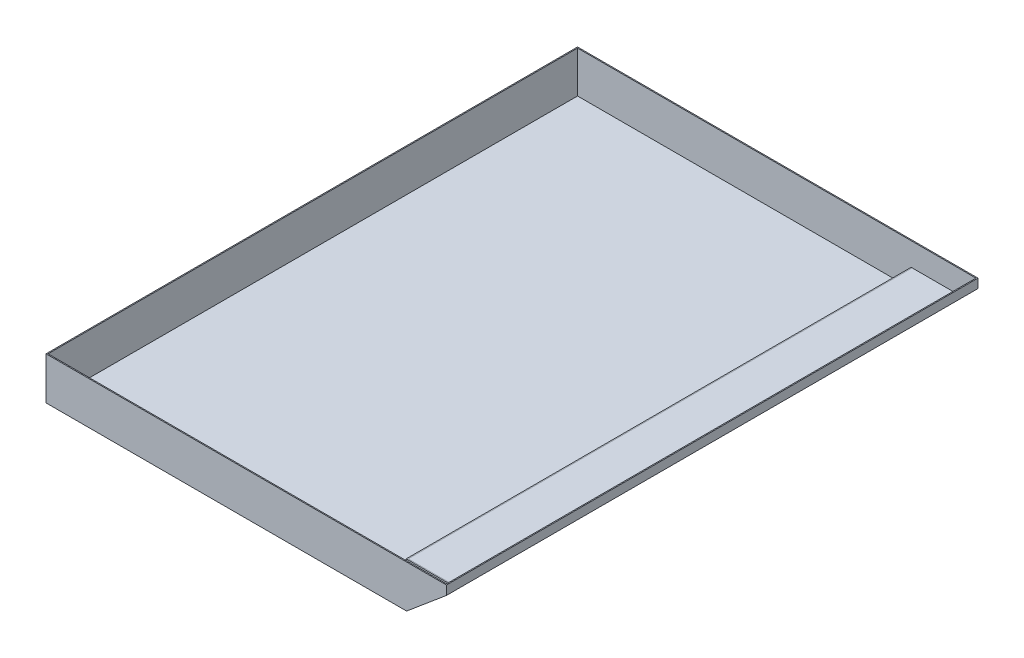
from build123d import *

# Parameters (mm, degrees)
EXTRUDE_1_DEPTH      = 1038
SKETCH_8_W           = 110.00435438
SKETCH_8_H           = 134.15256119
CUT_EXTRUDE_2_DEPTH  = 1191
SHELL_1_T            = -2
SKETCH_3_W           = 75
SKETCH_3_H           = 982
CUT_EXTRUDE_1_DEPTH  = 654
SKETCH_5_W           = 2
SKETCH_5_H           = 986
EXTRUDE_2_DEPTH      = 60
EXTRUDE_3_DEPTH      = 493
EXTRUDE_3_DEPTH_BACK = 493
EXTRUDE_5_DEPTH      = 2
EXTRUDE_6_DEPTH      = 2


with BuildPart() as part:
    # 草图2 → 凸台-拉伸1 (new body)
    with BuildSketch(Plane.XY):
        Polygon((0, 0), (0, 83), (784, 83), (784, 67), (704.152509296, 0), align=None)
    extrude(amount=EXTRUDE_1_DEPTH)

    # 草图8 → 切除-拉伸2 (cut)
    with BuildSketch(Plane.XY.offset(1038)):
        with Locations((837.00217719, 67.076280595)):
            Rectangle(SKETCH_8_W, SKETCH_8_H)
    extrude(amount=-CUT_EXTRUDE_2_DEPTH, mode=Mode.SUBTRACT)

    # 抽壳1
    shell_1_openings = [part.faces().sort_by_distance(p)[0] for p in [
        (391, 83, 519),
    ]]
    offset(amount=SHELL_1_T, openings=shell_1_openings, kind=Kind.INTERSECTION)

    # 草图3 → 切除-拉伸1 (cut)
    with BuildSketch(Plane(origin=(290.938854629, -346.727425229, 0), x_dir=(0.7660444431189772, 0.6427876096865405, 0), z_dir=(0.6427876096865404, -0.7660444431189772, 0))):
        with Locations((590.223457765, 519)):
            Rectangle(SKETCH_3_W, SKETCH_3_H)
    extrude(amount=-CUT_EXTRUDE_1_DEPTH, mode=Mode.SUBTRACT)

    # 草图5 → 凸台-拉伸2 (add)
    with BuildSketch(Plane(origin=(0, 2, 0), x_dir=(1, 0, 0), z_dir=(0, 1, 0))):
        with Locations((678.424568828, -519)):
            Rectangle(SKETCH_5_W, SKETCH_5_H)
    extrude(amount=EXTRUDE_2_DEPTH)


with BuildPart() as body_2:
    # 草图6 → 凸台-拉伸3 (new, two sides: drawn at the far end of the back side and taken through both)
    with BuildSketch(Plane.XY.offset(519).offset(-EXTRUDE_3_DEPTH_BACK)):
        Polygon((679.424568828, 62), (774.929784383, 62), (772.546277198, 60), (681.424568828, 60), (681.424568828, 4), (702.696628359, 4), (746.250437533, 40.545985214), (747.536012752, 39.013896328), (703.424568828, 2), (679.424568828, 2), align=None)
    extrude(amount=EXTRUDE_3_DEPTH + EXTRUDE_3_DEPTH_BACK)


with BuildPart() as body_3:
    # 草图9 → 凸台-拉伸5 (new body)
    with BuildSketch(Plane.XY.offset(1012)):
        Polygon((679.424568828, 62), (679.424568828, 2), (703.424568828, 2), (774.929784383, 62), align=None)
    extrude(amount=-EXTRUDE_5_DEPTH)


with BuildPart() as body_4:
    # 草图10 → 凸台-拉伸6 (new body)
    with BuildSketch(Plane(origin=(0, 0, 26), x_dir=(-1, 0, 0), z_dir=(0, 0, -1))):
        Polygon((-679.424568828, 2), (-679.424568828, 62), (-774.929784383, 62), (-703.424568828, 2), align=None)
    extrude(amount=-EXTRUDE_6_DEPTH)


solid = Compound([part.part, body_2.part, body_3.part, body_4.part])
